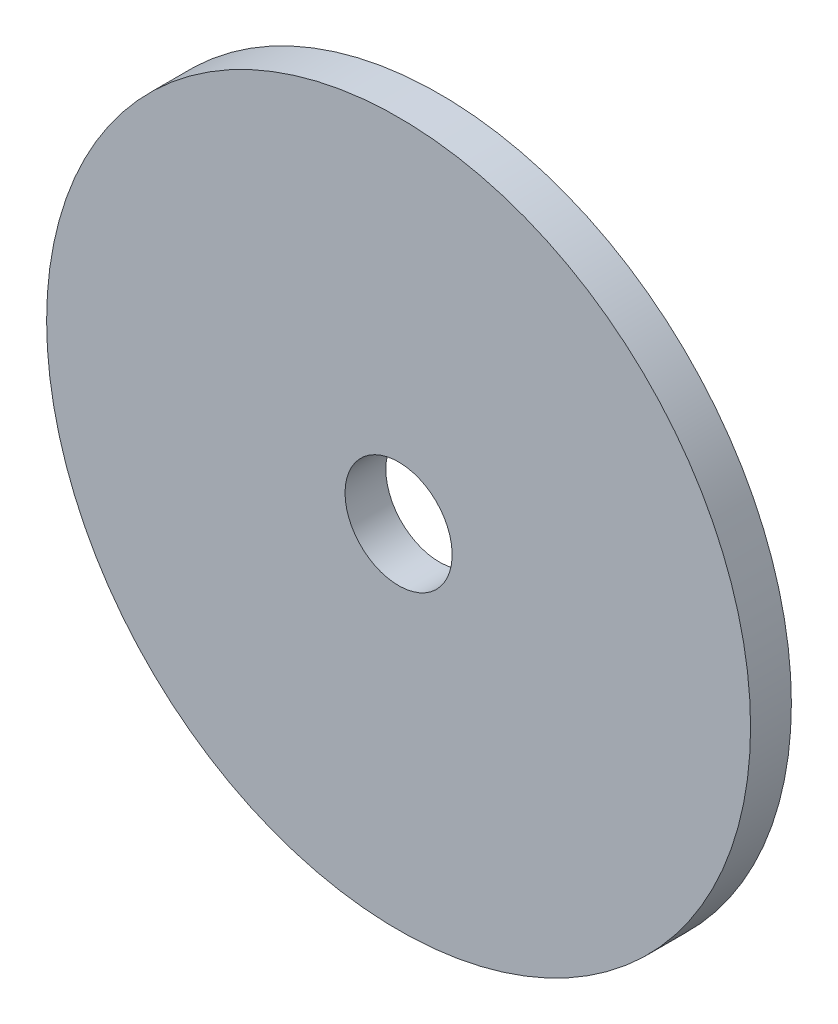
SolidWorks part; units mm, degrees
material "Q235"
ref_plane "Front Plane" through (0, 0, 0) normal (0, 0, 1) x (1, 0, 0)
ref_plane "Top Plane" through (0, 0, 0) normal (0, 1, 0) x (1, 0, 0)
ref_plane "Right Plane" through (0, 0, 0) normal (1, 0, 0) x (0, 0, -1)
sketch "Sketch1" plane through (0, 0, 0) normal (0, 0, 1) x (1, 0, 0)
  circle A0 centre (0, 0) radius 345
  dimension "D1" = 690
extrude "Boss-Extrude1" add sketch "Sketch1" along normal blind 40
sketch "Sketch8" plane through (0, 0, 40) normal (0, 0, -1) x (-1, 0, 0)
  circle A0 centre (0, 0) radius 52.5
  dimension "D1" = 105
extrude "Cut-Extrude3" cut sketch "Sketch8" against normal through all and the other way through all
